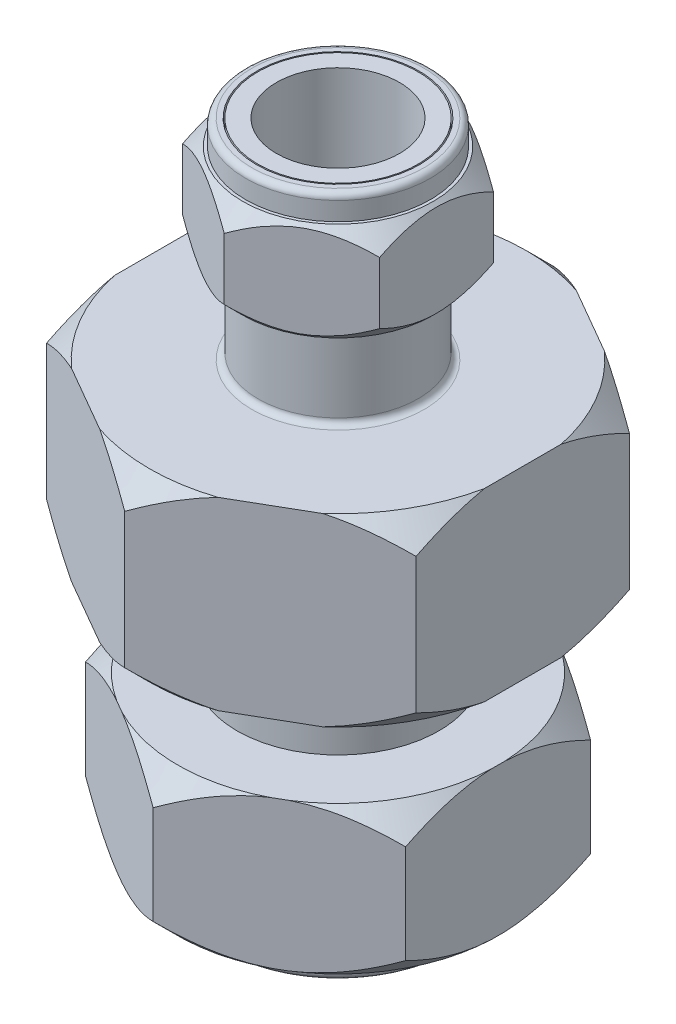
SolidWorks part; units mm, degrees
ref_plane "Front Plane" through (0, 0, 0) normal (0, 0, 1) x (1, 0, 0)
ref_plane "Top Plane" through (0, 0, 0) normal (0, 1, 0) x (1, 0, 0)
ref_plane "Right Plane" through (0, 0, 0) normal (1, 0, 0) x (0, 0, -1)
sketch "Sketch1" plane through (0, 0, 0) normal (0, 1, 0) x (1, 0, 0)
  line L1 (0, -17.3205) -> (15, -8.6603)
  line L2 (15, -8.6603) -> (15, 8.6603)
  line L3 (15, 8.6603) -> (0, 17.3205)
  line L4 (0, 17.3205) -> (-15, 8.6603)
  line L5 (-15, 8.6603) -> (-15, -8.6603)
  line L6 (-15, -8.6603) -> (0, -17.3205)
  circle A0 centre (0, 0) radius 15 construction
  dimension "D1" = 30
extrude "Boss-Extrude1" add sketch "Sketch1" along normal blind 15
sketch "Sketch2" plane through (0, 15, 0) normal (0, 1, 0) x (1, 0, 0)
  circle A0 centre (0, 0) radius 6.5
  dimension "D1" = 13
extrude "Boss-Extrude2" add sketch "Sketch2" along normal blind 17
sketch "Sketch3" plane through (0, 0, 0) normal (0, -1, 0) x (1, 0, 0)
  circle A0 centre (0, 0) radius 8
  dimension "D1" = 16
extrude "Boss-Extrude3" add sketch "Sketch3" along normal blind 22
sketch "Sketch4" plane through (0, -22, 0) normal (0, -1, 0) x (1, 0, 0)
  circle A0 centre (0, 0) radius 6.5
  dimension "D1" = 13
extrude "Cut-Extrude1" cut sketch "Sketch4" against normal blind 20
sketch "Sketch5" plane through (0, 32, 0) normal (0, 1, 0) x (1, 0, 0)
  circle A0 centre (0, 0) radius 5
  dimension "D1" = 10
extrude "Cut-Extrude2" cut sketch "Sketch5" against normal through all
sketch "Sketch6" plane through (0, 32, 0) normal (0, 1, 0) x (1, 0, 0)
  circle A0 centre (0, 0) radius 7.5
  circle A1 centre (0, 0) radius 6.6
  dimension "D1" = 15
  dimension "D2" = 13.2
extrude "Boss-Extrude4" add sketch "Sketch6" against normal blind 2 separate body
sketch "Sketch7" plane through (0, 30, 0) normal (0, -1, 0) x (1, 0, 0)
  line L1 (0, 9.2376) -> (-8, 4.6188)
  line L2 (-8, 4.6188) -> (-8, -4.6188)
  line L3 (-8, -4.6188) -> (0, -9.2376)
  line L4 (0, -9.2376) -> (8, -4.6188)
  line L5 (8, -4.6188) -> (8, 4.6188)
  line L6 (8, 4.6188) -> (0, 9.2376)
  circle A0 centre (0, 0) radius 6.6 construction
  circle A1 centre (0, 0) radius 6.6
  circle A2 centre (0, 0) radius 8 construction
  dimension "D1" = 16
extrude "Boss-Extrude5" add sketch "Sketch7" along normal blind 8
sketch "Sketch11" plane through (0, -22, 0) normal (0, -1, 0) x (1, 0, 0)
  circle A0 centre (0, 0) radius 9.5
  circle A3 centre (0, 0) radius 8.2
  circle A4 centre (0, 0) radius 8 construction
  dimension "D1" = 19
  dimension "D2" = 0.2
extrude "Boss-Extrude6" add sketch "Sketch11" against normal blind 3 separate body
sketch "Sketch12" plane through (0, -19, 0) normal (0, 1, 0) x (1, 0, 0)
  line L1 (0, 15.0111) -> (-13, 7.5056)
  line L2 (-13, 7.5056) -> (-13, -7.5056)
  line L3 (-13, -7.5056) -> (0, -15.0111)
  line L4 (0, -15.0111) -> (13, -7.5056)
  line L5 (13, -7.5056) -> (13, 7.5056)
  line L6 (13, 7.5056) -> (0, 15.0111)
  circle A0 centre (0, 0) radius 8.2 construction
  circle A1 centre (0, 0) radius 8.2
  circle A2 centre (0, 0) radius 13 construction
  dimension "D1" = 26
extrude "Boss-Extrude7" add sketch "Sketch12" along normal blind 12
sketch "Sketch9" plane through (0, 0, 0) normal (1, 0, 0) x (0, 0, -1)
  line L0 (-7.7376, 30) -> (-9.2376, 28.5)
  line L1 (-4.6188, 30) -> (-9.2376, 30) construction
  line L2 (-9.2376, 22) -> (-9.2376, 30) construction
  line L3 (-9.2376, 28.5) -> (-9.2376, 30)
  line L4 (-9.2376, 30) -> (-7.7376, 30)
  line L5 (-9.2376, 26) -> (-0.6273, 26) construction
  line L6 (-9.2376, 22) -> (-7.7376, 22)
  line L7 (-9.2376, 23.5) -> (-9.2376, 22)
  line L8 (-7.7376, 22) -> (-9.2376, 23.5)
  line L9 (0, 32) -> (0, 37.7244) construction
  line L10 (7.5, 32) -> (-7.5, 32) construction
  line L11 (-17.3205, 15) -> (-17.3205, 13)
  line L12 (-17.3205, 15) -> (-17.3205, 0) construction
  line L13 (-17.3205, 13) -> (-15.3205, 15)
  line L14 (-15.3205, 15) -> (-17.3205, 15)
  line L15 (-17.3205, 7.5) -> (-4.5484, 7.5) construction
  line L16 (-15.3205, 0) -> (-17.3205, 0)
  line L17 (-17.3205, 2) -> (-15.3205, 0)
  line L18 (-17.3205, 0) -> (-17.3205, 2)
  line L19 (-15.0111, -13) -> (3.4609, -13) construction
  line L20 (-15.0111, -7) -> (-15.0111, -19) construction
  line L21 (-15.0111, -7) -> (-15.0111, -9)
  line L22 (-15.0111, -7) -> (-7.5056, -7) construction
  line L23 (-15.0111, -9) -> (-13.0111, -7)
  line L24 (-13.0111, -7) -> (-15.0111, -7)
  line L25 (-13.0111, -19) -> (-15.0111, -19)
  line L26 (-15.0111, -17) -> (-13.0111, -19)
  line L27 (-15.0111, -19) -> (-15.0111, -17)
  dimension "D1" = 1.5
  dimension "D2" = 2
revolve "Cut-Revolve2" cut sketch "Sketch9" angle 360 about L9
fillet "Fillet1" radius 0.5 1 edges at (0, 32, 7.5)
fillet "Fillet2" radius 0.5 2 edges at (0, 0, -8) (0, 15, 6.5)
fillet "Fillet3" radius 0.5 1 edges at (0, -22, -9.5)
